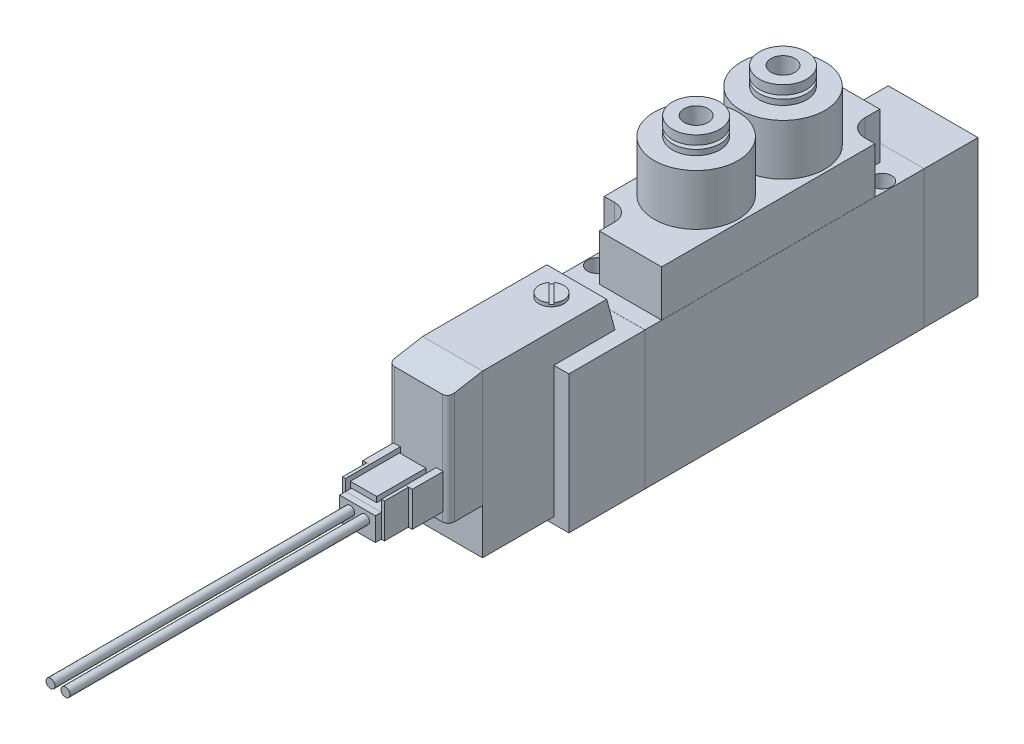
from build123d import *

# Parameters (mm, degrees)
SKETCH_1_W           = 46.6
SKETCH_1_H           = 23
EXTRUDE_1_DEPTH      = 15
SKETCH_2_W           = 14.98
SKETCH_2_H           = 22.98
EXTRUDE_2_DEPTH      = 9
SKETCH_3_W           = 14.98
SKETCH_3_H           = 22.98
EXTRUDE_3_DEPTH      = 0.01
SKETCH_7_W           = 12.71
SKETCH_7_H           = 22.98
EXTRUDE_4_DEPTH      = 0.01
SKETCH_8_W           = 12.71
SKETCH_8_H           = 22.98
EXTRUDE_5_DEPTH      = 15.01
EXTRUDE_6_DEPTH      = 5
EXTRUDE_6_DEPTH_BACK = 5
EXTRUDE_7_DEPTH      = 19.45
CUT_EXTRUDE_1_DEPTH  = 15
SKETCH_12_W          = 6
SKETCH_12_H          = 2.26
EXTRUDE_8_DEPTH      = 5.15
SKETCH_13_W          = 6
SKETCH_13_H          = 2.26
EXTRUDE_9_DEPTH      = 0.01
EXTRUDE_10_DEPTH     = 4
EXTRUDE_11_DEPTH     = 6
SKETCH_16_W          = 0.4
SKETCH_16_H          = 0.4
EXTRUDE_12_DEPTH     = 1.5
SKETCH_17_W          = 0.4
SKETCH_17_H          = 0.4
EXTRUDE_13_DEPTH     = 0.01
SKETCH_18_W          = 0.4
SKETCH_18_H          = 0.4
EXTRUDE_14_DEPTH     = 1.5
SKETCH_19_W          = 0.4
SKETCH_19_H          = 0.4
EXTRUDE_15_DEPTH     = 0.01
SKETCH_20_W          = 4.4
SKETCH_20_H          = 8.2
EXTRUDE_16_DEPTH     = 0.9
SKETCH_21_W          = 5.98
SKETCH_21_H          = 3.88
EXTRUDE_17_DEPTH     = 1
SKETCH_22_W          = 5.98
SKETCH_22_H          = 3.88
EXTRUDE_18_DEPTH     = 0.01
SKETCH_23_R          = 0.75
EXTRUDE_19_DEPTH     = 50
EXTRUDE_START        = -0.01
SKETCH_24_R          = 0.75
EXTRUDE_20_DEPTH     = 0.01
SKETCH_25_R          = 0.75
EXTRUDE_21_DEPTH     = 50
SKETCH_26_R          = 0.75
EXTRUDE_22_DEPTH     = 0.01
SKETCH_27_R          = 2.075
EXTRUDE_23_DEPTH     = 0.6
SKETCH_28_R          = 2.075
EXTRUDE_24_DEPTH     = 0.01
CUT_EXTRUDE_3_DEPTH  = 0.25
SKETCH_31_W          = 14.98
SKETCH_31_H          = 41
EXTRUDE_25_DEPTH     = 7.7
SKETCH_32_W          = 14.98
SKETCH_32_H          = 41
EXTRUDE_26_DEPTH     = 0.01
CUT_EXTRUDE_4_DEPTH  = 8.7
CUT_EXTRUDE_5_DEPTH  = 8.7
SKETCH_37_R          = 2
CUT_EXTRUDE_6_DEPTH  = 20.2
SKETCH_38_R          = 2
CUT_EXTRUDE_7_DEPTH  = 20.2
SKETCH_41_R          = 1.6
CUT_EXTRUDE_8_DEPTH  = 523


with BuildPart() as part:
    # 草图1 → 拉伸1 (new body)
    with BuildSketch(Plane(origin=(0, 0, 0), x_dir=(0, 0, -1), z_dir=(1, 0, 0))):
        with Locations((23.3, 11.5)):
            Rectangle(SKETCH_1_W, SKETCH_1_H)
    extrude(amount=-EXTRUDE_1_DEPTH)

    # 草图2 → 拉伸2 (add)
    with BuildSketch(Plane(origin=(0, 0, -46.6), x_dir=(-1, 0, 0), z_dir=(0, 0, -1))):
        with Locations((7.5, 11.5)):
            Rectangle(SKETCH_2_W, SKETCH_2_H)
    extrude(amount=EXTRUDE_2_DEPTH)

    # 草图3 → 拉伸3 (add)
    with BuildSketch(Plane(origin=(0, 0, -46.6), x_dir=(-1, 0, 0), z_dir=(0, 0, -1))):
        with Locations((7.5, 11.5)):
            Rectangle(SKETCH_3_W, SKETCH_3_H)
    extrude(amount=-EXTRUDE_3_DEPTH)

    # 草图4 → 切除-旋转1 (revolve, cut)
    with BuildSketch(Plane(origin=(-7.5, 0, 0), x_dir=(0, 0, -1), z_dir=(1, 0, 0))):
        Polygon((23.3, 8), (27.585, 8), (27.585, 0.5), (28.585, -0.5), (23.3, -0.5), align=None)
    revolve(axis=Axis((-7.5, -0.5, -23.3), (0, 1, 0)), mode=Mode.SUBTRACT)

    # 草图5 → 切除-旋转2 (revolve, cut)
    with BuildSketch(Plane(origin=(-6.7, 0, 0), x_dir=(0, 0, -1), z_dir=(1, 0, 0))):
        Polygon((9.7, 8), (13.985, 8), (13.985, 0.5), (14.985, -0.5), (9.7, -0.5), align=None)
    revolve(axis=Axis((-6.7, -0.5, -9.7), (0, 1, 0)), mode=Mode.SUBTRACT)

    # 草图6 → 切除-旋转3 (revolve, cut)
    with BuildSketch(Plane(origin=(-8.3, 0, 0), x_dir=(0, 0, -1), z_dir=(1, 0, 0))):
        Polygon((36.9, 8), (41.185, 8), (41.185, 0.5), (42.185, -0.5), (36.9, -0.5), align=None)
    revolve(axis=Axis((-8.3, -0.5, -36.9), (0, 1, 0)), mode=Mode.SUBTRACT)

    # 草图7 → 拉伸4 (add)
    with BuildSketch(Plane(origin=(0, 0, 0), x_dir=(0, 0, -1), z_dir=(1, 0, 0))):
        with Locations((-6.345, 11.5)):
            Rectangle(SKETCH_7_W, SKETCH_7_H)
    extrude(amount=EXTRUDE_4_DEPTH)

    # 草图8 → 拉伸5 (add)
    with BuildSketch(Plane(origin=(0, 0, 0), x_dir=(0, 0, -1), z_dir=(1, 0, 0))):
        with Locations((-6.345, 11.5)):
            Rectangle(SKETCH_8_W, SKETCH_8_H)
    extrude(amount=-EXTRUDE_5_DEPTH)

    # 草图9 → 拉伸6 (add, two sides: drawn at the far end of the back side and taken through both)
    with BuildSketch(Plane(origin=(-7.5, 0, 0), x_dir=(0, 0, -1), z_dir=(1, 0, 0)).offset(-EXTRUDE_6_DEPTH_BACK)):
        Polygon((-24.6, 1.1), (-12.7, 1.1), (-12.7, 0.01), (-2.5, 0.01), (-2.5, 23), (-3.866540881, 28.1), (-24.6, 28.1), align=None)
    extrude(amount=EXTRUDE_6_DEPTH + EXTRUDE_6_DEPTH_BACK)

    # 草图10 → 拉伸7 (add)
    with BuildSketch(Plane(origin=(0, 28.1, 0), x_dir=(-1, 0, 0), z_dir=(0, 1, 0))):
        with BuildLine():
            Line((12.49, 24.59), (12.49, 29.3))
            ThreePointArc((12.49, 29.3), (12.197106781, 30.007106781), (11.49, 30.3))
            Line((11.49, 30.3), (3.51, 30.3))
            ThreePointArc((3.51, 30.3), (2.802893219, 30.007106781), (2.51, 29.3))
            Line((2.51, 29.3), (2.51, 24.59))
            Line((2.51, 24.59), (12.49, 24.59))
        make_face()
    extrude(amount=-EXTRUDE_7_DEPTH)

    # 草图11 → 切除-拉伸1 (cut)
    with BuildSketch(Plane(origin=(0, 0, 0), x_dir=(0, 0, -1), z_dir=(1, 0, 0))):
        Polygon((-34.6, 26.336730193), (-13.257436361, 30.1), (-34.6, 30.1), align=None)
    extrude(amount=-CUT_EXTRUDE_1_DEPTH, mode=Mode.SUBTRACT)

    # 草图12 → 拉伸8 (add)
    with BuildSketch(Plane.XY.offset(30.3)):
        Polygon((-3.37, 10.2), (-3.37, 16), (-4.51, 16), (-4.51, 14.1), (-10.51, 14.1), (-10.51, 16), (-11.65, 16), (-11.65, 10.2), align=None)
        with Locations((-7.51, 12.47)):
            Rectangle(SKETCH_12_W, SKETCH_12_H, mode=Mode.SUBTRACT)
    extrude(amount=EXTRUDE_8_DEPTH)

    # 草图13 → 拉伸9 (add)
    with BuildSketch(Plane.XY.offset(30.3)):
        Polygon((-3.37, 10.2), (-3.37, 16), (-4.51, 16), (-4.51, 14.1), (-10.51, 14.1), (-10.51, 16), (-11.65, 16), (-11.65, 10.2), align=None)
        with Locations((-7.51, 12.47)):
            Rectangle(SKETCH_13_W, SKETCH_13_H, mode=Mode.SUBTRACT)
    extrude(amount=-EXTRUDE_9_DEPTH)

    # 草图14 → 拉伸10 (add)
    with BuildSketch(Plane.XY.offset(35.45)):
        Polygon((-11.01, 15.99), (-11.01, 10.21), (-4.01, 10.21), (-4.01, 15.99), (-4.51, 15.99), (-4.51, 14.09), (-10.51, 14.09), (-10.51, 15.99), align=None)
    extrude(amount=EXTRUDE_10_DEPTH)

    # 草图15 → 拉伸11 (add)
    with BuildSketch(Plane.XY.offset(35.45)):
        Polygon((-11.01, 15.99), (-11.01, 10.21), (-4.01, 10.21), (-4.01, 15.99), (-4.51, 15.99), (-4.51, 14.09), (-10.51, 14.09), (-10.51, 15.99), align=None)
    extrude(amount=-EXTRUDE_11_DEPTH)

    # 草图16 → 拉伸12 (add)
    with BuildSketch(Plane(origin=(0, 14.09, 0), x_dir=(-1, 0, 0), z_dir=(0, 1, 0))):
        with Locations((5.51, 36.15)):
            Rectangle(SKETCH_16_W, SKETCH_16_H)
    extrude(amount=EXTRUDE_12_DEPTH)

    # 草图17 → 拉伸13 (add)
    with BuildSketch(Plane(origin=(0, 14.09, 0), x_dir=(-1, 0, 0), z_dir=(0, 1, 0))):
        with Locations((5.51, 36.15)):
            Rectangle(SKETCH_17_W, SKETCH_17_H)
    extrude(amount=-EXTRUDE_13_DEPTH)

    # 草图18 → 拉伸14 (add)
    with BuildSketch(Plane(origin=(0, 14.09, 0), x_dir=(-1, 0, 0), z_dir=(0, 1, 0))):
        with Locations((9.51, 36.15)):
            Rectangle(SKETCH_18_W, SKETCH_18_H)
    extrude(amount=EXTRUDE_14_DEPTH)

    # 草图19 → 拉伸15 (add)
    with BuildSketch(Plane(origin=(0, 14.09, 0), x_dir=(-1, 0, 0), z_dir=(0, 1, 0))):
        with Locations((9.51, 36.15)):
            Rectangle(SKETCH_19_W, SKETCH_19_H)
    extrude(amount=-EXTRUDE_15_DEPTH)

    # 草图20 → 拉伸16 (add)
    with BuildSketch(Plane(origin=(0, 15.99, 0), x_dir=(-1, 0, 0), z_dir=(0, 1, 0))):
        with Locations((7.51, 35.35)):
            Rectangle(SKETCH_20_W, SKETCH_20_H)
    extrude(amount=-EXTRUDE_16_DEPTH)

    # 草图21 → 拉伸17 (add)
    with BuildSketch(Plane.XY.offset(39.45)):
        with Locations((-7.51, 12.16)):
            Rectangle(SKETCH_21_W, SKETCH_21_H)
    extrude(amount=EXTRUDE_17_DEPTH)

    # 草图22 → 拉伸18 (add)
    with BuildSketch(Plane.XY.offset(39.45)):
        with Locations((-7.51, 12.16)):
            Rectangle(SKETCH_22_W, SKETCH_22_H)
    extrude(amount=-EXTRUDE_18_DEPTH)

    # 草图23 → 拉伸19 (add)
    with BuildSketch(Plane.XY.offset(40.45)):
        with Locations((-8.75, 12.75)):
            Circle(SKETCH_23_R)
    extrude(amount=EXTRUDE_19_DEPTH)

    # 草图24 → 拉伸20 (add)
    with BuildSketch(Plane.XY.offset(40.45).offset(EXTRUDE_START)):
        with Locations((-8.75, 12.75)):
            Circle(SKETCH_24_R)
    extrude(amount=EXTRUDE_20_DEPTH)

    # 草图25 → 拉伸21 (add)
    with BuildSketch(Plane.XY.offset(40.45)):
        with Locations((-6.25, 12.75)):
            Circle(SKETCH_25_R)
    extrude(amount=EXTRUDE_21_DEPTH)

    # 草图26 → 拉伸22 (add)
    with BuildSketch(Plane.XY.offset(40.45).offset(EXTRUDE_START)):
        with Locations((-6.25, 12.75)):
            Circle(SKETCH_26_R)
    extrude(amount=EXTRUDE_22_DEPTH)

    # 草图27 → 拉伸23 (add)
    with BuildSketch(Plane(origin=(0, 28.1, 0), x_dir=(-1, 0, 0), z_dir=(0, 1, 0))):
        with Locations(Location((7.5, 8.1, 0), (0, 0, 270))):
            Circle(SKETCH_27_R)
    extrude(amount=EXTRUDE_23_DEPTH)

    # 草图28 → 拉伸24 (add)
    with BuildSketch(Plane(origin=(0, 28.1, 0), x_dir=(-1, 0, 0), z_dir=(0, 1, 0)).offset(EXTRUDE_START)):
        with Locations(Location((7.5, 8.1, 0), (0, 0, 270))):
            Circle(SKETCH_28_R)
    extrude(amount=EXTRUDE_24_DEPTH)

    # 草图30 → 切除-拉伸3 (cut)
    with BuildSketch(Plane(origin=(0, 28.7, 0), x_dir=(-1, 0, 0), z_dir=(0, 1, 0))):
        with BuildLine():
            Line((5.81817412, 9.357561811), (8.757561811, 6.41817412))
            ThreePointArc((8.757561811, 6.41817412), (8.98492424, 6.61507576), (9.18182588, 6.842438189))
            Line((9.18182588, 6.842438189), (6.242438189, 9.78182588))
            ThreePointArc((6.242438189, 9.78182588), (6.01507576, 9.58492424), (5.81817412, 9.357561811))
        make_face()
    extrude(amount=-CUT_EXTRUDE_3_DEPTH, mode=Mode.SUBTRACT)

    # 草图31 → 拉伸25 (add)
    with BuildSketch(Plane(origin=(0, 23, 0), x_dir=(-1, 0, 0), z_dir=(0, 1, 0))):
        with Locations((7.5, -23.3)):
            Rectangle(SKETCH_31_W, SKETCH_31_H)
    extrude(amount=EXTRUDE_25_DEPTH)

    # 草图32 → 拉伸26 (add)
    with BuildSketch(Plane(origin=(0, 23, 0), x_dir=(-1, 0, 0), z_dir=(0, 1, 0))):
        with Locations((7.5, -23.3)):
            Rectangle(SKETCH_32_W, SKETCH_32_H)
    extrude(amount=-EXTRUDE_26_DEPTH)

    # 草图33 → 切除-拉伸4 (cut)
    with BuildSketch(Plane(origin=(0, 23, 0), x_dir=(-1, 0, 0), z_dir=(0, 1, 0))):
        with BuildLine():
            Line((4.6, -43.8), (4.6, -41.3))
            ThreePointArc((4.6, -41.3), (3.750609665, -39.249390335), (1.7, -38.4))
            Line((1.7, -38.4), (-2, -38.4))
            Line((-2, -38.4), (-2, -43.8))
            Line((-2, -43.8), (4.6, -43.8))
        make_face()
    extrude(amount=CUT_EXTRUDE_4_DEPTH, mode=Mode.SUBTRACT)

    # 草图34 → 切除-拉伸5 (cut)
    with BuildSketch(Plane(origin=(0, 23, 0), x_dir=(-1, 0, 0), z_dir=(0, 1, 0))):
        with BuildLine():
            Line((16, -2.8), (10.4, -2.8))
            Line((10.4, -2.8), (10.4, -5.3))
            ThreePointArc((10.4, -5.3), (11.249390335, -7.350609665), (13.3, -8.2))
            Line((13.3, -8.2), (16, -8.2))
            Line((16, -8.2), (16, -2.8))
        make_face()
    extrude(amount=CUT_EXTRUDE_5_DEPTH, mode=Mode.SUBTRACT)

    # 草图35 → 旋转1 (revolve)
    with BuildSketch(Plane(origin=(-7.5, 0, 0), x_dir=(0, 0, -1), z_dir=(1, 0, 0)), mode=Mode.PRIVATE) as revolve_1_sk:
        Polygon((16.05, 42.2), (20, 42.2), (20, 40.7), (18.25, 40.7), (18.25, 40.1), (20, 40.1), (20, 39.2), (23.05, 39.2), (23.05, 30.69), (16.05, 30.69), align=None)
    revolve(revolve_1_sk.sketch.rotate(Axis((-7.5, 30.69, -16.05), (0, 1, 0)), 180), axis=Axis((-7.5, 30.69, -16.05), (0, 1, 0)))

    # 草图36 → 旋转2 (revolve)
    with BuildSketch(Plane(origin=(-7.5, 0, 0), x_dir=(0, 0, -1), z_dir=(1, 0, 0)), mode=Mode.PRIVATE) as revolve_2_sk:
        Polygon((30.55, 42.2), (34.5, 42.2), (34.5, 40.7), (32.75, 40.7), (32.75, 40.1), (34.5, 40.1), (34.5, 39.2), (37.55, 39.2), (37.55, 30.69), (30.55, 30.69), align=None)
    revolve(revolve_2_sk.sketch.rotate(Axis((-7.5, 30.69, -30.55), (0, 1, 0)), 180), axis=Axis((-7.5, 30.69, -30.55), (0, 1, 0)))

    # 草图37 → 切除-拉伸6 (cut)
    with BuildSketch(Plane(origin=(0, 42.2, 0), x_dir=(-1, 0, 0), z_dir=(0, 1, 0))):
        with Locations(Location((7.5, -16.05, 0), (0, 0, 90))):
            Circle(SKETCH_37_R)
    extrude(amount=-CUT_EXTRUDE_6_DEPTH, mode=Mode.SUBTRACT)

    # 草图38 → 切除-拉伸7 (cut)
    with BuildSketch(Plane(origin=(0, 42.2, 0), x_dir=(-1, 0, 0), z_dir=(0, 1, 0))):
        with Locations(Location((7.5, -30.55, 0), (0, 0, 90))):
            Circle(SKETCH_38_R)
    extrude(amount=-CUT_EXTRUDE_7_DEPTH, mode=Mode.SUBTRACT)

    # 草图39 → 切除-旋转4 (revolve, cut)
    with BuildSketch(Plane(origin=(0, 16.7, 0), x_dir=(-1, 0, 0), z_dir=(0, 1, 0)), mode=Mode.PRIVATE) as cut_revolve_4_sk:
        Polygon((15.5, -34.6), (15.5, -36.83), (14.5, -35.83), (8.5, -35.83), (8.5, -34.6), align=None)
    revolve(cut_revolve_4_sk.sketch.rotate(Axis((-8.5, 16.7, -34.6), (-1, 0, 0)), 180), axis=Axis((-8.5, 16.7, -34.6), (-1, 0, 0)), mode=Mode.SUBTRACT)

    # 草图40 → 切除-旋转5 (revolve, cut)
    with BuildSketch(Plane(origin=(0, 16.7, 0), x_dir=(-1, 0, 0), z_dir=(0, 1, 0)), mode=Mode.PRIVATE) as cut_revolve_5_sk:
        Polygon((15.5, -12), (15.5, -14.23), (14.5, -13.23), (8.5, -13.23), (8.5, -12), align=None)
    revolve(cut_revolve_5_sk.sketch.rotate(Axis((-8.5, 16.7, -12), (-1, 0, 0)), 180), axis=Axis((-8.5, 16.7, -12), (-1, 0, 0)), mode=Mode.SUBTRACT)

    # 草图41 → 切除-拉伸8 (cut)
    with BuildSketch(Plane(origin=(0, 30.7, 0), x_dir=(1, 0, 0), z_dir=(0, 1, 0))):
        with Locations(Location((-13.3, 5.3, 0), (0, 0, 270))):
            Circle(SKETCH_41_R)
        with Locations(Location((-1.7, 41.3, 0), (0, 0, 270))):
            Circle(SKETCH_41_R)
    extrude(amount=-CUT_EXTRUDE_8_DEPTH, mode=Mode.SUBTRACT)


solid = part.part
